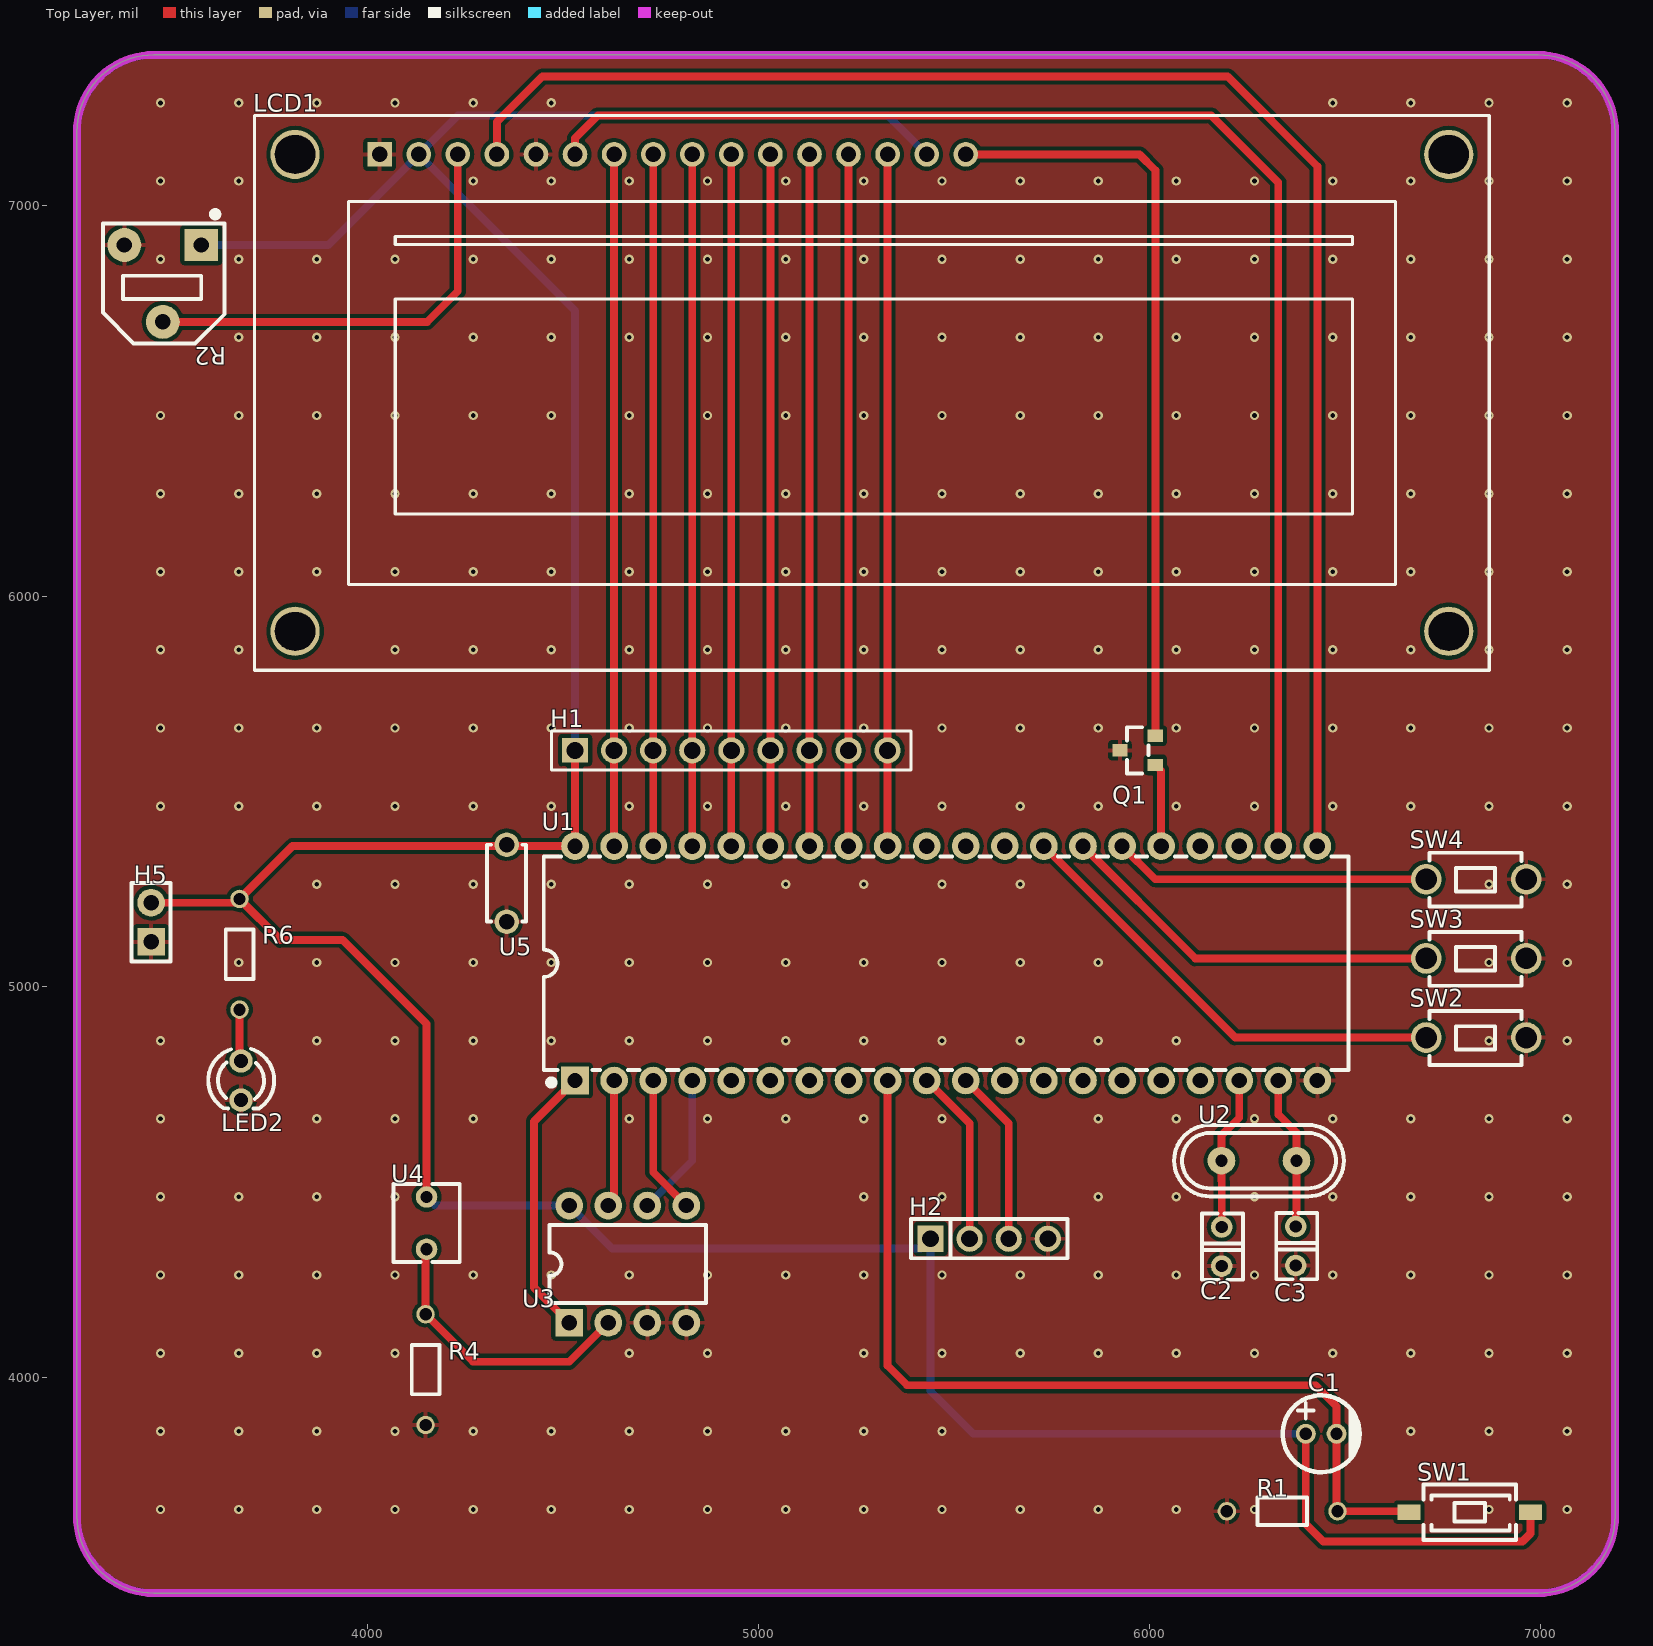
[diagram p0: Top Layer view]
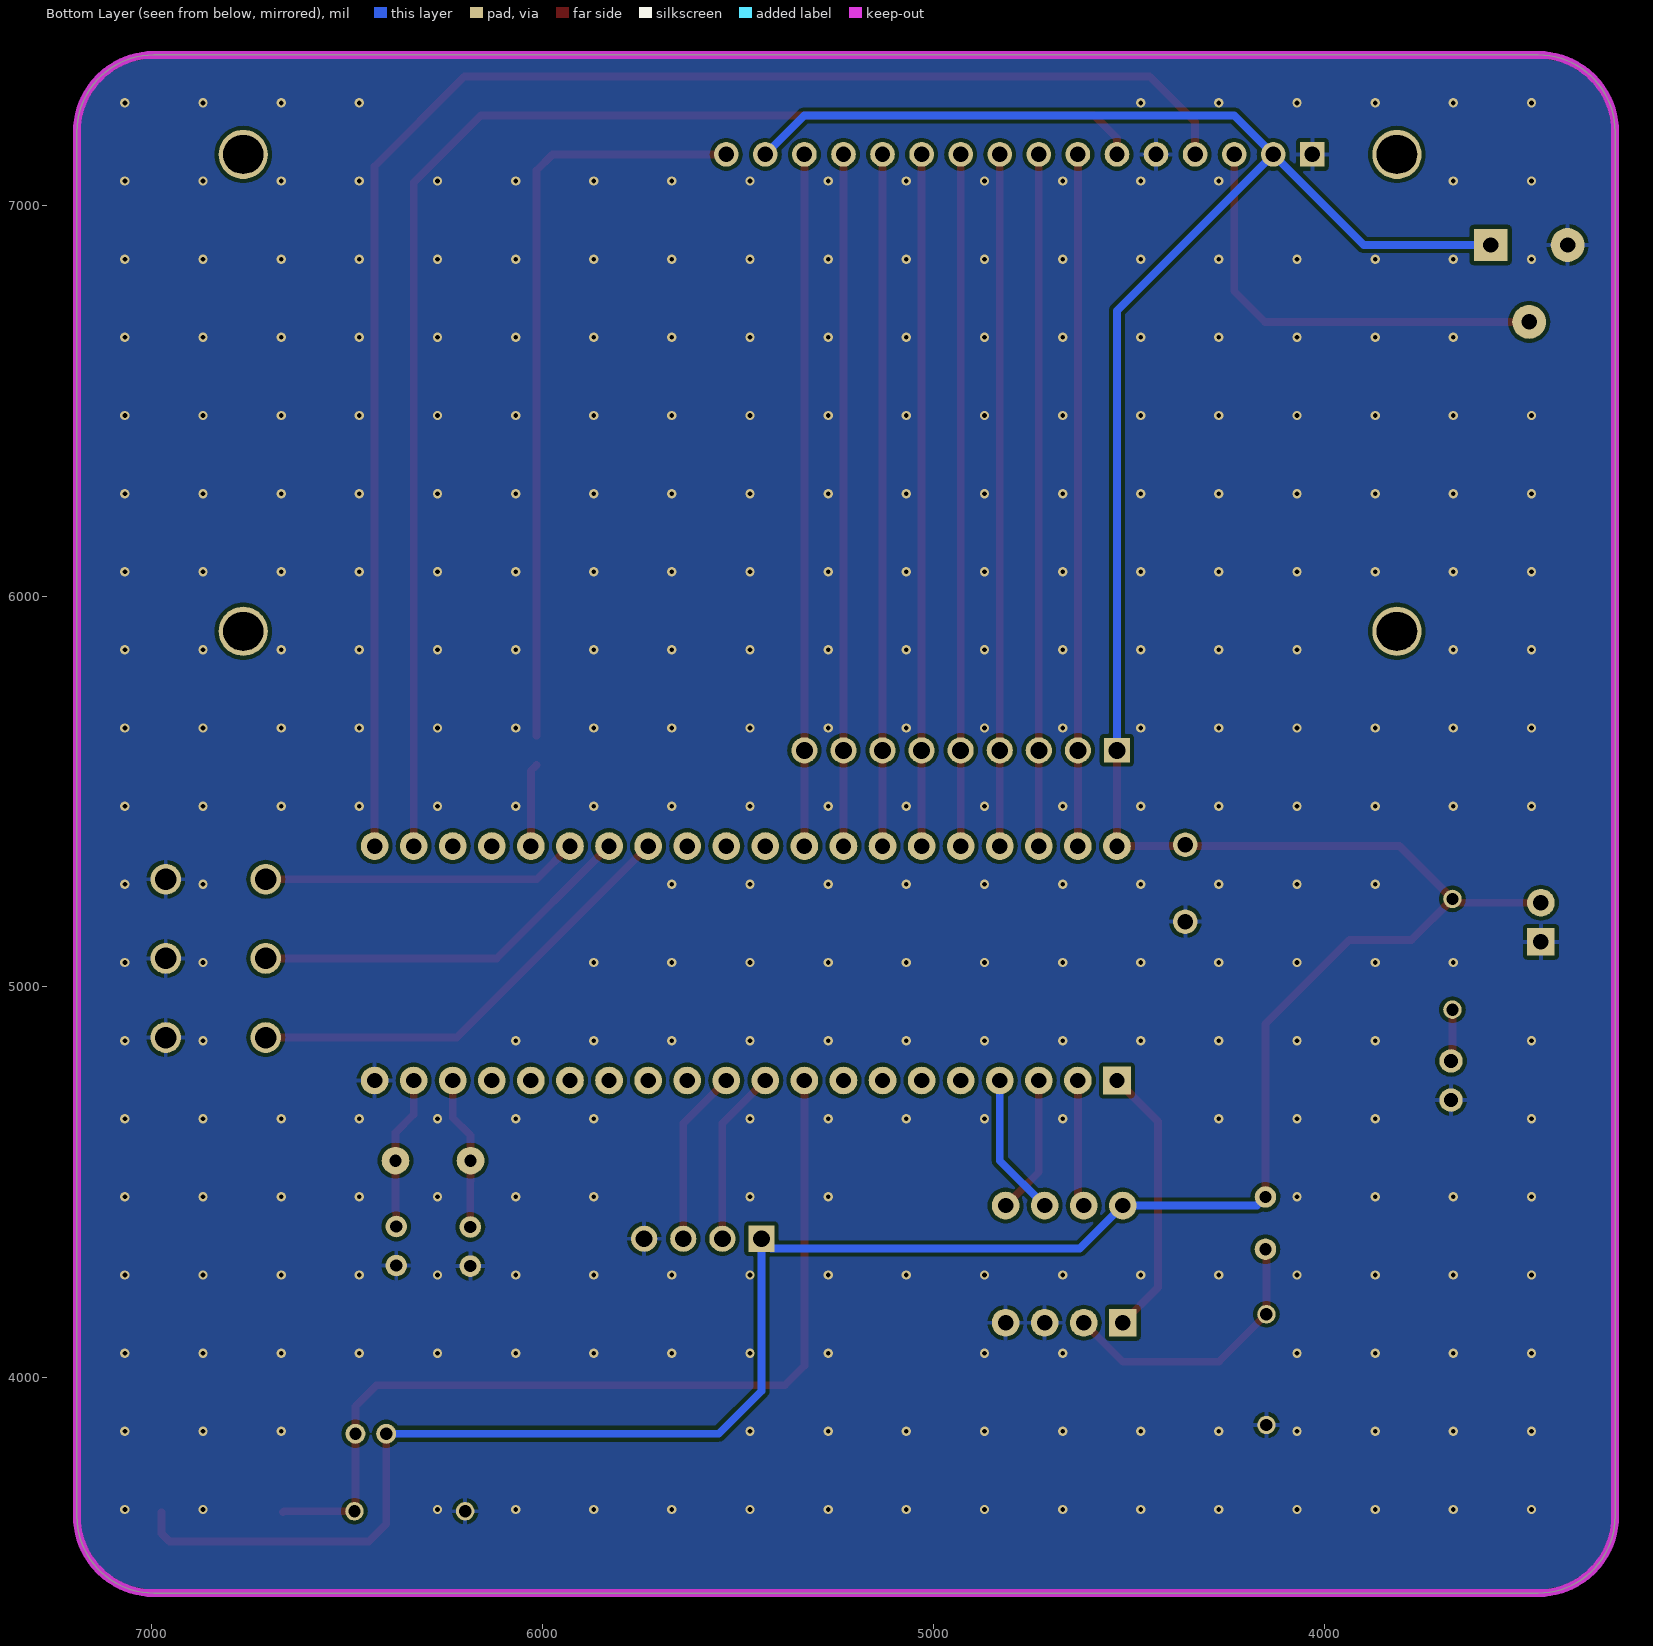
[diagram p1: Bottom Layer view, seen from below]
# Altium PCB MISC51926.pcbdoc
Units mil, origin at the board's own origin, x right, y up, seen from the top; angles counter-clockwise.
Board outline 3937.01 x 3937.01 mil, 2 copper layers (Top Layer, Bottom Layer), stack 62.206 mil thick; 22 components, 29 nets, 117 pads, 313 vias.

## Layer stack, top to bottom
Top Solder Mask Layer: solder mask 0.394, Dk 3.3
Top Layer: signal copper 1.379
Dielectric1: surface 59.449, FR4, Dk 4.5
Bottom Layer: signal copper 1.378
Bottom Solder Mask Layer: solder mask 0.394, Dk 3.3

## Board outline
3451.85,7385 ccw(c3451.85,7188.15) 3255,7188.15 3255,3644.84 ccw(c3451.85,3644.84) 3451.85,3447.99 6995.16,3447.99 ccw(c6995.16,3644.84) 7192.01,3644.84 7192.01,7188.15 ccw(c6995.16,7188.15) 6995.16,7385

## Design rules (kind name [scope] priority, off if disabled: settings)
BoardOutlineClearance copperThickness2oz_1 [All] p2 off: genericclearance=7.99 ignorepadtopadclearanceinfootprint=FALSE except(0: Arc-SplitContinuation Track-SplitContinuation SMDPad-SplitContinuation THPad-SplitContinuation Via-SplitContinuation Fill-SplitContinuation Region-SplitContinuation Poly-SplitContinuation Text-SplitContinuation Hole-SplitContinuation; 5.98: Arc-CutoutEdge Track-CutoutEdge SMDPad-CutoutEdge THPad-CutoutEdge Via-CutoutEdge Text-CutoutEdge; 6.9: Hole-OutlineEdge Hole-CutoutEdge; 10: Poly-OutlineEdge Poly-CutoutEdge; 11.81: Arc-OutlineEdge Track-OutlineEdge SMDPad-OutlineEdge THPad-OutlineEdge Via-OutlineEdge Fill-OutlineEdge Region-OutlineEdge Text-OutlineEdge Fill-CutoutEdge Region-CutoutEdge)
BoardOutlineClearance Plane_innerPlane_1 [All] p4 off: genericclearance=4.02 ignorepadtopadclearanceinfootprint=FALSE except(0: Arc-SplitContinuation Track-SplitContinuation SMDPad-SplitContinuation THPad-SplitContinuation Via-SplitContinuation Fill-SplitContinuation Region-SplitContinuation Poly-SplitContinuation Text-SplitContinuation Hole-SplitContinuation; 5.98: Arc-CutoutEdge Track-CutoutEdge SMDPad-CutoutEdge THPad-CutoutEdge Via-CutoutEdge Text-CutoutEdge; 6.9: Hole-OutlineEdge Hole-CutoutEdge; 10: Poly-OutlineEdge Poly-CutoutEdge; 11.81: Arc-OutlineEdge Track-OutlineEdge SMDPad-OutlineEdge THPad-OutlineEdge Via-OutlineEdge Fill-OutlineEdge Region-OutlineEdge Text-OutlineEdge Fill-CutoutEdge Region-CutoutEdge)
BoardOutlineClearance Copper_copperRegion_1 [All] p6 off: genericclearance=4.02 ignorepadtopadclearanceinfootprint=FALSE except(0: Arc-SplitContinuation Track-SplitContinuation SMDPad-SplitContinuation THPad-SplitContinuation Via-SplitContinuation Fill-SplitContinuation Region-SplitContinuation Poly-SplitContinuation Text-SplitContinuation Hole-SplitContinuation; 5.98: Arc-CutoutEdge Track-CutoutEdge SMDPad-CutoutEdge THPad-CutoutEdge Via-CutoutEdge Text-CutoutEdge; 6.9: Hole-OutlineEdge Hole-CutoutEdge; 10: Poly-OutlineEdge Poly-CutoutEdge; 11.81: Arc-OutlineEdge Track-OutlineEdge SMDPad-OutlineEdge THPad-OutlineEdge Via-OutlineEdge Fill-OutlineEdge Region-OutlineEdge Text-OutlineEdge Fill-CutoutEdge Region-CutoutEdge)
BoardOutlineClearance copperThickness1oz_1 [All] p8: genericclearance=4.02 ignorepadtopadclearanceinfootprint=FALSE except(0: Arc-SplitContinuation Track-SplitContinuation SMDPad-SplitContinuation THPad-SplitContinuation Via-SplitContinuation Fill-SplitContinuation Region-SplitContinuation Poly-SplitContinuation Text-SplitContinuation Hole-SplitContinuation; 5.98: Arc-CutoutEdge Track-CutoutEdge SMDPad-CutoutEdge THPad-CutoutEdge Via-CutoutEdge Text-CutoutEdge; 6.9: Hole-OutlineEdge Hole-CutoutEdge; 10: Poly-OutlineEdge Poly-CutoutEdge; 11.81: Arc-OutlineEdge Track-OutlineEdge SMDPad-OutlineEdge THPad-OutlineEdge Via-OutlineEdge Fill-OutlineEdge Region-OutlineEdge Text-OutlineEdge Fill-CutoutEdge Region-CutoutEdge)
Clearance copperThickness2oz [All] p1 off: gap=7.99 ignorepadtopadclearanceinfootprint=FALSE except(5.98: SMDPad-Track SMDPad-SMDPad THPad-Track SMDPad-THPad THPad-THPad Track-Via SMDPad-Via THPad-Via Via-Via Fill-SMDPad Region-SMDPad Fill-THPad Region-THPad Fill-Via Region-Via Fill-Fill Fill-Region Region-Region Arc-Track Arc-SMDPad Arc-THPad Arc-Via Fill-Arc Region-Arc Arc-Arc Text-Track SMDPad-Text Text-THPad Text-Via Fill-Text Region-Text Arc-Text Text-Text; 6.9: Hole-Track Hole-SMDPad Hole-THPad Hole-Via Fill-Hole Region-Hole Hole-Arc Hole-Text; 10: Poly-Track Poly-SMDPad Poly-THPad Poly-Via Poly-Fill Poly-Region Poly-Poly Poly-Arc Poly-Text Poly-Hole; 11.81: Fill-Track Region-Track)
Clearance Plane_innerPlane [All] p3 off: gap=4.02 ignorepadtopadclearanceinfootprint=FALSE except(5.98: SMDPad-Track SMDPad-SMDPad THPad-Track SMDPad-THPad THPad-THPad Track-Via SMDPad-Via THPad-Via Via-Via Fill-SMDPad Region-SMDPad Fill-THPad Region-THPad Fill-Via Region-Via Fill-Fill Fill-Region Region-Region Arc-Track Arc-SMDPad Arc-THPad Arc-Via Fill-Arc Region-Arc Arc-Arc Text-Track SMDPad-Text Text-THPad Text-Via Fill-Text Region-Text Arc-Text Text-Text; 6.9: Hole-Track Hole-SMDPad Hole-THPad Hole-Via Fill-Hole Region-Hole Hole-Arc Hole-Text; 10: Poly-Track Poly-SMDPad Poly-THPad Poly-Via Poly-Fill Poly-Region Poly-Poly Poly-Arc Poly-Text Poly-Hole; 11.81: Fill-Track Region-Track)
Clearance Copper_copperRegion [All] p5 off: gap=4.02 ignorepadtopadclearanceinfootprint=FALSE except(5.98: SMDPad-Track SMDPad-SMDPad THPad-Track SMDPad-THPad THPad-THPad Track-Via SMDPad-Via THPad-Via Via-Via Fill-SMDPad Region-SMDPad Fill-THPad Region-THPad Fill-Via Region-Via Fill-Fill Fill-Region Region-Region Arc-Track Arc-SMDPad Arc-THPad Arc-Via Fill-Arc Region-Arc Arc-Arc Text-Track SMDPad-Text Text-THPad Text-Via Fill-Text Region-Text Arc-Text Text-Text; 6.9: Hole-Track Hole-SMDPad Hole-THPad Hole-Via Fill-Hole Region-Hole Hole-Arc Hole-Text; 10: Poly-Track Poly-SMDPad Poly-THPad Poly-Via Poly-Fill Poly-Region Poly-Poly Poly-Arc Poly-Text Poly-Hole; 11.81: Fill-Track Region-Track)
Clearance copperThickness1oz [All] p7: gap=4.02 ignorepadtopadclearanceinfootprint=FALSE except(5.98: SMDPad-Track SMDPad-SMDPad THPad-Track SMDPad-THPad THPad-THPad Track-Via SMDPad-Via THPad-Via Via-Via Fill-SMDPad Region-SMDPad Fill-THPad Region-THPad Fill-Via Region-Via Fill-Fill Fill-Region Region-Region Arc-Track Arc-SMDPad Arc-THPad Arc-Via Fill-Arc Region-Arc Arc-Arc Text-Track SMDPad-Text Text-THPad Text-Via Fill-Text Region-Text Arc-Text Text-Text; 6.9: Hole-Track Hole-SMDPad Hole-THPad Hole-Via Fill-Hole Region-Hole Hole-Arc Hole-Text; 10: Poly-Track Poly-SMDPad Poly-THPad Poly-Via Poly-Fill Poly-Region Poly-Poly Poly-Arc Poly-Text Poly-Hole; 11.81: Fill-Track Region-Track)
DiffPairsRouting differentialPair [All] p1: maxlimit=6 minlimit=6 mostfreqgap=6 toplayer_minwidth=5 toplayer_prefwidth=10 toplayer_maxwidth=100 toplayer_mingap=6 toplayer_prefgap=6 toplayer_maxgap=6 bottomlayer_minwidth=5 bottomlayer_prefwidth=10 bottomlayer_maxwidth=100 bottomlayer_mingap=6 bottomlayer_prefgap=6 bottomlayer_maxgap=6 maxuncoupledlength=10
HoleToHoleClearance otherClearance [All] p1: gap=11.81 allowstackedmicrovias=TRUE
Length netLength [All] p1: minlimit=0 maxlimit=0
PasteMaskExpansion pasteMaskExpansion [All] p1: expansion=0
PlaneConnect innerPlane [All] p1: planeconnectstyle=Relief reliefexpansion=20 reliefentries=4 reliefconductorwidth=10 reliefairgap=10
PolygonConnect copperRegion [All] p1: connectstyle=Relief reliefconductorwidth=10 reliefentries=4 polygonreliefangle="90 Angle" airgapwidth=10 via.connectstyle=Relief via.reliefconductorwidth=10 via.reliefentries=4 via.polygonreliefangle="90 Angle" via.airgapwidth=10
RoutingVias viaSize [All] p1: holewidth=12.01 width=24.02 viastyle="Through Hole" minholewidth=11.81 minwidth=19.68 maxholewidth=248.03 maxwidth=393.7
SolderMaskExpansion solderMaskExpansion [IsVia] p1: expansion=-1000 istentingtop=TRUE
SolderMaskExpansion solderMaskExpansion [All] p2: expansion=2 istentingtop=FALSE
Width copperThickness2oz_2 [All] p1 off: maxlimit=100 minlimit=8 preferedwidth=10
Width copperThickness1oz_2 [All] p2: maxlimit=100 minlimit=5 preferedwidth=10

## Components (designator, comment, footprint, x,y, rotation, side; value= is the part's Value field where it differs from the comment)
C1 "10uF" CAP-TH_BD5.0-P2.00-D0.8-FD-10UF50VC110GL 6439.62,3855.84 r0 top
C2 "30pF" CAP-TH_L3.8-W2.5-P2.54-D0.50 6185,4335 r90 top
C3 "30pF" CAP-TH_L3.8-W2.5-P2.54-D0.50 6374.59,4336.33 r90 top
H1 "" HDR-TH_9P-P2.54-V-F-1 4930,5605 r0 top
H2 "" HDR-TH_4P-P2.54-V-M 5590,4355 r0 top
H5 "" HDR-TH_2P-P2.54-V-M-1 3445,5165 r90 top
LCD1 "LMB162ADC" LCD1602 5289.84,6520 r0 top
LED2 "" LED_TH-3mm 3675,4760 r270 top
Q1 "" S8050_SOT-23 5970,5605 r0 top
R1 "10kΩ" Res_1/8W 6340,3655 r0 top
R2 "10kΩ" RES-ADJ-SMD_RM065-V1 3475,6800 r180 top
R4 "10kΩ" Res_1/8W 4150,4020 r90 top
R6 "220Ω" Res_1/8W 3673.87,5083.05 r90 top
SW1 "Tact switch 3*6*2.5" SW-SMD_L6.0-W3.6-LS8.0 6820,3655 r0 top
SW2 "" Key_TH_3.5x6x4.3 6830,4870 r0 top
SW3 "" Key_TH_3.5x6x4.3 6830,5072.5 r0 top
SW4 "" Key_TH_3.5x6x4.3 6830,5275 r0 top
U1 "STC89C516RD+40I-PDIP40" DIP-40_L52.3-W13.9-P2.54-LS15.2-BL 5480,5060 r0 top
U2 "11.0592MHz" HC-49US_L11.0-W4.6-P4.88 6280.51,4554.79 r0 top
U3 "ADC0832CCN" DIP-8_L9.7-W6.4-P2.54-LS7.6-BL 4665,4290 r0 top
U4 "光敏电阻-5MM" RES-TH_L4.9-W4.3-P3.4 4150,4395 r270 top
U5 "100nF" CAP-TH_L5.0-W2.5-P5.00-D1.0 4355,5265 r270 top

## Footprints (in the part's own frame and the unit in brackets; to place one, negate y for a bottom-side part, rotate by r counter-clockwise, add the part's x,y. Pads: shape width x height; smd on the part's side, far side on the other; paste and mask are expansions set on the pad)
CAP-TH_BD5.0-P2.00-D0.8-FD-10UF50VC110GL [mm]
  round 1.3 hole 0.8: 1(-1,0) 2(1,0)
  silkscreen extent -2.5,-2.5 2.5,2.5
CAP-TH_L3.8-W2.5-P2.54-D0.50 [mm]
  round 1.4 hole 0.8 paste+0 mask+0.05: 1(-1.27,0) 2(1.27,0)
  silkscreen extent -2.16,-1.4 2.16,1.27
CAP-TH_L5.0-W2.5-P5.00-D1.0 [mm]
  round 1.6 hole 1: 1(-2.5,0) 2(2.5,0)
  silkscreen extent -2.5,-1.27 2.5,1.25
DIP-8_L9.7-W6.4-P2.54-LS7.6-BL [mm]
  rect 1.8x1.8 hole 1 paste+0 mask+0.05: 1(-3.81,-3.81)
  round 1.8 hole 1 paste+0 mask+0.05: 2(-1.27,-3.81) 3(1.27,-3.81) 4(3.81,-3.81) 5(3.81,3.81) 6(1.27,3.81) 7(-1.27,3.81) 8(-3.81,3.81)
  silkscreen extent -5.08,-2.53 5.08,2.53
DIP-40_L52.3-W13.9-P2.54-LS15.2-BL [mm]
  rect 1.8x1.8 hole 1: 1(-24.13,-7.62)
  round 1.8 hole 1: 2(-21.59,-7.62) 3(-19.05,-7.62) 4(-16.51,-7.62) 5(-13.97,-7.62) 6(-11.43,-7.62) 7(-8.89,-7.62) 8(-6.35,-7.62) 9(-3.81,-7.62) 10(-1.27,-7.62) 11(1.27,-7.62) 12(3.81,-7.62) 13(6.35,-7.62) 14(8.89,-7.62) 15(11.43,-7.62) 16(13.97,-7.62) 17(16.51,-7.62) 18(19.05,-7.62) 19(21.59,-7.62) 20(24.13,-7.62) 21(24.13,7.62) 22(21.59,7.62) 23(19.05,7.62) 24(16.51,7.62) 25(13.97,7.62) 26(11.43,7.62) 27(8.89,7.62) 28(6.35,7.62) 29(3.81,7.62) 30(1.27,7.62) 31(-1.27,7.62) 32(-3.81,7.62) 33(-6.35,7.62) 34(-8.89,7.62) 35(-11.43,7.62) 36(-13.97,7.62) 37(-16.51,7.62) 38(-19.05,7.62) 39(-21.59,7.62) 40(-24.13,7.62)
  silkscreen extent -26.16,-7.95 26.16,6.93
HC-49US_L11.0-W4.6-P4.88 [mm]
  round 1.8 hole 0.8: 1(-2.44,0) 2(2.44,0)
  silkscreen extent -5.51,-2.32 5.51,2.32
HDR-TH_2P-P2.54-V-M-1 [mm]
  rect 1.8x1.8 hole 1: 1(-1.27,0)
  round 1.8 hole 1: 2(1.27,0)
  silkscreen extent -2.54,-1.27 2.54,1.27
HDR-TH_4P-P2.54-V-M [mm]
  rect 1.7x1.7 hole 1.1: 1(-3.81,0)
  round 1.7 hole 1.1: 2(-1.27,0) 3(1.27,0) 4(3.81,0)
  silkscreen extent -5.08,-1.27 5.08,1.27
HDR-TH_9P-P2.54-V-F-1 [mm]
  rect 1.7x1.575 hole 1.1: 1(-10.16,0)
  round 1.7 hole 1.1: 2(-7.62,0) 3(-5.08,0) 4(-2.54,0) 5(0,0) 6(2.54,0) 7(5.08,0) 8(7.62,0) 9(10.16,0)
  silkscreen extent -11.68,-1.27 11.68,1.27
Key_TH_3.5x6x4.3 [mil]
  round 78.7 hole 55.1 paste+0 mask+2: A(-121.44,0) B(134.46,0)
  silkscreen extent -114,-70 123,68
LCD1602 [mm]
  round 3.2 hole 2.5 slot 2.625 at 0 deg: 0(-37.5,-15.5) 0(-37.5,15.5) 0(37.5,-15.5) 0(37.5,15.5)
  rect 1.6x1.6 hole 1: 1(-32,15.5)
  round 1.6 hole 1: 2(-29.46,15.5) 3(-26.92,15.5) 4(-24.38,15.5) 5(-21.84,15.5) 6(-19.3,15.5) 7(-16.76,15.5) 8(-14.22,15.5) 9(-11.68,15.5) 10(-9.14,15.5) 11(-6.6,15.5) 12(-4.06,15.5) 13(-1.52,15.5) 14(1.02,15.5) 15(3.56,15.5) 16(6.1,15.5)
  silkscreen extent -40.13,-18.03 40.13,18.03
LED_TH-3mm [mil]
  round 60 hole 36 paste+0 mask+2: 1(-50,0) 2(50,0)
  silkscreen extent -81,-84 72,85
RES-ADJ-SMD_RM065-V1 [mm]
  rect 2.2x2.1 hole 1 paste+0 mask+0.05: 1(-2.5,-2.5)
  round 2.2 hole 1 paste+0 mask+0.05: 2(0,2.5) 3(2.5,-2.5)
  silkscreen extent -4,-4.7 3.9,3.9
RES-TH_L4.9-W4.3-P3.4 [mm]
  round 1.4 hole 0.8 paste+0 mask+0.05: 1(-1.7,0) 2(1.7,0)
  silkscreen extent -2.54,-2.16 2.54,2.16
Res_1/8W [mil]
  round 47.2 hole 31.5 paste+0 mask+2: 1(-141.7,2.48) 2(141.7,2.48)
  silkscreen extent -63,-33 63,38
S8050_SOT-23 [mm]
  rect 1x0.8 smd paste+0 mask+0.051: 1(1.15,-0.95) 2(1.15,0.95) 3(-1.15,0)
  silkscreen extent -0.7,-1.5 0.7,1.5
SW-SMD_L6.0-W3.6-LS8.0 [mm]
  rect 1.5x1 smd: 1(-3.95,0) 2(3.95,0)
  silkscreen extent -3,-1.8 3,1.8

## Via types
v1: diameter 24.02, hole 12, Top Layer to Bottom Layer, 313 vias

## Nets (pads, with @x,y where several pads share a name; then routed paths per layer and width w, separated by ;. In a path a pad name is that pad's centre, name@x,y a point inside that pad or via, vN(x,y) a via of type N, cw(c..) or ccw(c..) an arc to the next point about the centre after c; other vN are vias at no path point)
$1N504: H1.9 LCD1.14 U1.32 | length 1770.2
  Top Layer w20: U1.32 H1.9 LCD1.14
$1N506: H1.8 LCD1.13 U1.33 | length 1770.2
  Top Layer w20: U1.33 H1.8 LCD1.13
$1N508: H1.7 LCD1.12 U1.34 | length 1770.2
  Top Layer w20: U1.34 H1.7 LCD1.12
$1N510: H1.6 LCD1.11 U1.35 | length 1770.2
  Top Layer w20: U1.35 H1.6 LCD1.11
$1N512: H1.5 LCD1.10 U1.36 | length 1770.2
  Top Layer w20: U1.36 H1.5 LCD1.10
$1N514: H1.4 LCD1.9 U1.37 | length 1770.2
  Top Layer w20: U1.37 H1.4 LCD1.9
$1N516: H1.3 LCD1.8 U1.38 | length 1770.2
  Top Layer w20: U1.38 H1.3 LCD1.8
$1N518: H1.2 LCD1.7 U1.39 | length 1770.2
  Top Layer w20: U1.39 H1.2 LCD1.7
$1N1145: LCD1.3 R2.2 | length 1137.7
  Top Layer w20: R2.2 4151.57,6701.57 4230,6780 LCD1.3
$1N1588: C2.2 U1.18 U2.1 | length 394.1
  Top Layer w20: C2.2 6185,4503.47 6184.45,4504.02 6184.45,4554.79 6184.45,4619.45 6230,4665 U1.18
$1N1593: C3.2 U1.19 U2.2 | length 393.8
  Top Layer w20: U1.19 6330,4673.21 6376.57,4626.64 U2.2 6376.57,4425.87 6374.59,4423.89 C3.2
$1N2914: C1.2 R1.2 SW1.1 U1.9 | length 2375.5
  Top Layer w20: U1.9 5330,4030 5380,3980 6425,3980 6478.99,3926.01 C1.2 6478.99,3660.19 R1.2 6662.01,3657.48 SW1.1
$1N3621: LED2.1 R6.1 | length 132.8
  Top Layer w20: R6.1 3671.39,4813.61 LED2.1
$1N3773: U1.1 U3.1 | length 700.8
  Top Layer w20: U3.1 4425,4230 4425,4655 U1.1
$1N3774: R4.2 U3.2 U4.2 | length 726.7
  Top Layer w20: U4.2 4147.52,4325.59 R4.2 4269.22,4040 4515,4040 U3.2
$1N3779: U1.2 U3.7 | length 326.2
  Top Layer w20: U3.7 4630,4455 U1.2
$1N3780: U1.3 U3.5 | length 355.2
  Top Layer w20: U1.3 4730,4525 U3.5
$1N3781: U1.4 U3.6 | length 367.6
  Bottom Layer w20: U3.6 4830,4555 U1.4
$1N3791: LCD1.16 Q1.2 | length 1949.4
  Top Layer w20: LCD1.16 5974.76,7130.24 6015.28,7089.72 Q1.2
$1N3796: SW2.A U1.28 | length 1181.5
  Top Layer w20: U1.28 6220,4870 SW2.A
$1N3797: SW3.A U1.27 | length 997.6
  Top Layer w20: U1.27 6117.5,5072.5 SW3.A
$1N3798: SW4.A U1.26 | length 813.8
  Top Layer w20: U1.26 6015,5275 SW4.A
GND: C2.1 C3.1 H2.4 H5.1 LCD1.1 LCD1.5 LED2.2 Q1.3 R1.1 R2.3 R4.1 SW2.B SW3.B SW4.B U1.20 U3.3 U3.4 U5.2
  other v1: 3469.1,3662.09 3669.1,3662.09 3869.1,3662.09 4069.1,3662.09 4269.1,3662.09 4469.1,3662.09 4669.1,3662.09 4869.1,3662.09 5069.1,3662.09 5269.1,3662.09 5469.1,3662.09 5669.1,3662.09 5869.1,3662.09 6069.1,3662.09 6269.1,3662.09 6869.1,3662.09 7069.1,3662.09 3469.1,3862.09 3669.1,3862.09 3869.1,3862.09 4069.1,3862.09 4269.1,3862.09 4469.1,3862.09 4669.1,3862.09 4869.1,3862.09 5069.1,3862.09 5269.1,3862.09 5469.1,3862.09 6669.1,3862.09 6869.1,3862.09 7069.1,3862.09 3469.1,4062.09 3669.1,4062.09 3869.1,4062.09 4069.1,4062.09 4669.1,4062.09 4869.1,4062.09 5269.1,4062.09 5469.1,4062.09 5669.1,4062.09 5869.1,4062.09 6069.1,4062.09 6269.1,4062.09 6469.1,4062.09 6669.1,4062.09 6869.1,4062.09 7069.1,4062.09 3469.1,4262.09 3669.1,4262.09 3869.1,4262.09 4069.1,4262.09 4269.1,4262.09 4469.1,4262.09 4669.1,4262.09 4869.1,4262.09 5069.1,4262.09 5269.1,4262.09 5469.1,4262.09 5669.1,4262.09 5869.1,4262.09 6069.1,4262.09 6269.1,4262.09 6469.1,4262.09 6669.1,4262.09 6869.1,4262.09 7069.1,4262.09 3469.1,4462.09 3669.1,4462.09 3869.1,4462.09 4069.1,4462.09 5269.1,4462.09 5469.1,4462.09 5869.1,4462.09 6069.1,4462.09 6269.1,4462.09 6469.1,4462.09 6669.1,4462.09 6869.1,4462.09 7069.1,4462.09 3469.1,4662.09 3869.1,4662.09 4069.1,4662.09 4269.1,4662.09 4669.1,4662.09 4869.1,4662.09 5069.1,4662.09 5269.1,4662.09 5469.1,4662.09 5869.1,4662.09 6069.1,4662.09 6269.1,4662.09 6469.1,4662.09 6669.1,4662.09 6869.1,4662.09 7069.1,4662.09 3469.1,4862.09 3869.1,4862.09 4069.1,4862.09 4269.1,4862.09 4469.1,4862.09 4669.1,4862.09 4869.1,4862.09 5069.1,4862.09 5269.1,4862.09 5469.1,4862.09 5669.1,4862.09 5869.1,4862.09 6069.1,4862.09 6869.1,4862.09 7069.1,4862.09 3669.1,5062.09 3869.1,5062.09 4069.1,5062.09 4269.1,5062.09 4469.1,5062.09 4669.1,5062.09 4869.1,5062.09 5069.1,5062.09 5269.1,5062.09 5469.1,5062.09 5669.1,5062.09 5869.1,5062.09 6869.1,5062.09 7069.1,5062.09 3869.1,5262.09 4069.1,5262.09 4269.1,5262.09 4469.1,5262.09 4669.1,5262.09 4869.1,5262.09 5069.1,5262.09 5269.1,5262.09 5469.1,5262.09 5669.1,5262.09 6869.1,5262.09 7069.1,5262.09 3469.1,5462.09 3669.1,5462.09 3869.1,5462.09 4069.1,5462.09 4269.1,5462.09 4469.1,5462.09 4669.1,5462.09 4869.1,5462.09 5069.1,5462.09 5269.1,5462.09 5469.1,5462.09 5669.1,5462.09 5869.1,5462.09 6069.1,5462.09 6269.1,5462.09 6469.1,5462.09 6669.1,5462.09 6869.1,5462.09 7069.1,5462.09 3469.1,5662.09 3669.1,5662.09 3869.1,5662.09 4069.1,5662.09 4269.1,5662.09 4469.1,5662.09 4669.1,5662.09 4869.1,5662.09 5069.1,5662.09 5269.1,5662.09 5469.1,5662.09 5669.1,5662.09 5869.1,5662.09 6069.1,5662.09 6269.1,5662.09 6469.1,5662.09 6669.1,5662.09 6869.1,5662.09 7069.1,5662.09 3469.1,5862.09 3669.1,5862.09 4069.1,5862.09 4269.1,5862.09 4469.1,5862.09 4669.1,5862.09 4869.1,5862.09 5069.1,5862.09 5269.1,5862.09 5469.1,5862.09 5669.1,5862.09 5869.1,5862.09 6069.1,5862.09 6269.1,5862.09 6469.1,5862.09 6669.1,5862.09 6869.1,5862.09 7069.1,5862.09 3469.1,6062.09 3669.1,6062.09 3869.1,6062.09 4069.1,6062.09 4269.1,6062.09 4469.1,6062.09 4669.1,6062.09 4869.1,6062.09 5069.1,6062.09 5269.1,6062.09 5469.1,6062.09 5669.1,6062.09 5869.1,6062.09 6069.1,6062.09 6269.1,6062.09 6469.1,6062.09 6669.1,6062.09 6869.1,6062.09 7069.1,6062.09 3469.1,6262.09 3669.1,6262.09 3869.1,6262.09 4069.1,6262.09 4269.1,6262.09 4469.1,6262.09 4669.1,6262.09 4869.1,6262.09 5069.1,6262.09 5269.1,6262.09 5469.1,6262.09 5669.1,6262.09 5869.1,6262.09 6069.1,6262.09 6269.1,6262.09 6469.1,6262.09 6669.1,6262.09 6869.1,6262.09 7069.1,6262.09 3469.1,6462.09 3669.1,6462.09 3869.1,6462.09 4069.1,6462.09 4269.1,6462.09 4469.1,6462.09 4669.1,6462.09 4869.1,6462.09 5069.1,6462.09 5269.1,6462.09 5469.1,6462.09 5669.1,6462.09 5869.1,6462.09 6069.1,6462.09 6269.1,6462.09 6469.1,6462.09 6669.1,6462.09 6869.1,6462.09 7069.1,6462.09 3669.1,6662.09 3869.1,6662.09 4069.1,6662.09 4269.1,6662.09 4469.1,6662.09 4669.1,6662.09 4869.1,6662.09 5069.1,6662.09 5269.1,6662.09 5469.1,6662.09 5669.1,6662.09 5869.1,6662.09 6069.1,6662.09 6269.1,6662.09 6469.1,6662.09 6669.1,6662.09 6869.1,6662.09 7069.1,6662.09 3469.1,6862.09 3669.1,6862.09 3869.1,6862.09 4069.1,6862.09 4269.1,6862.09 4469.1,6862.09 4669.1,6862.09 4869.1,6862.09 5069.1,6862.09 5269.1,6862.09 5469.1,6862.09 5669.1,6862.09 5869.1,6862.09 6069.1,6862.09 6269.1,6862.09 6469.1,6862.09 6669.1,6862.09 6869.1,6862.09 7069.1,6862.09 3469.1,7062.09 3669.1,7062.09 4269.1,7062.09 4469.1,7062.09 4669.1,7062.09 4869.1,7062.09 5069.1,7062.09 5269.1,7062.09 5469.1,7062.09 5669.1,7062.09 5869.1,7062.09 6069.1,7062.09 6269.1,7062.09 6469.1,7062.09 6669.1,7062.09 6869.1,7062.09 7069.1,7062.09 3469.1,7262.09 3669.1,7262.09 3869.1,7262.09 4069.1,7262.09 4269.1,7262.09 4469.1,7262.09 6469.1,7262.09 6669.1,7262.09 6869.1,7262.09 7069.1,7262.09
L1: LCD1.6 U1.22 | length 3635.2
  Top Layer w20: LCD1.6 4530,7171.74 4588.26,7230 6158.58,7230 6330,7058.58 U1.22
L2: LCD1.4 U1.21 | length 4066.6
  Top Layer w20: LCD1.4 4330,7213.16 4446.84,7330 6200,7330 6430,7100 U1.21
PWM: Q1.1 U1.25 | length 213.7
  Top Layer w20: Q1.1 6030,5552.87 U1.25
RXD: H2.2 U1.10 | length 450.6
  Top Layer w20: U1.10 5540,4650 H2.2
TXD: H2.3 U1.11 | length 450.6
  Top Layer w20: U1.11 5640,4650 H2.3
VCC: C1.1 H1.1 H2.1 H5.2 LCD1.2 LCD1.15 R2.1 R6.2 SW1.2 U1.40 U3.8 U4.1 U5.1 | length 9808.7
  Top Layer w20: H5.2 3661.64,5215 R6.2 ; U4.1 4150,4905 3935,5120 3776.14,5120 R6.2 ; H1.1 U1.40 3806.64,5360 R6.2 ; C1.1 6400.25,3624.75 6445,3580 6955,3580 6975.51,3600.51 SW1.2
  Bottom Layer w20: R2.1 3898.18,6898.43 LCD1.2 ; U4.1 4171.93,4440 U3.8 4625,4330 5415,4330 H2.1 5440,3965 5549.16,3855.84 C1.1 ; H1.1 4530,6730.24 LCD1.2 ; LCD1.15 5330.24,7230 4229.76,7230 LCD1.2
pads on no net: LCD1.0 U1.5 U1.6 U1.7 U1.8 U1.12 U1.13 U1.14 U1.15 U1.16 U1.17 U1.23 U1.24 U1.29 U1.30 U1.31

## Polygon pours and split planes (outlines as drawn)
GND on Top Layer (solid, remove dead copper, pour order 0): 3000,7595 3000,3000 7325,3000 7325,7595
GND on Bottom Layer (solid, remove dead copper, pour order 2): 3075,7640 3075,3120 7710,3120 7710,7640

## Keep-outs
Board Outline Layer:
  the board outline again, w20